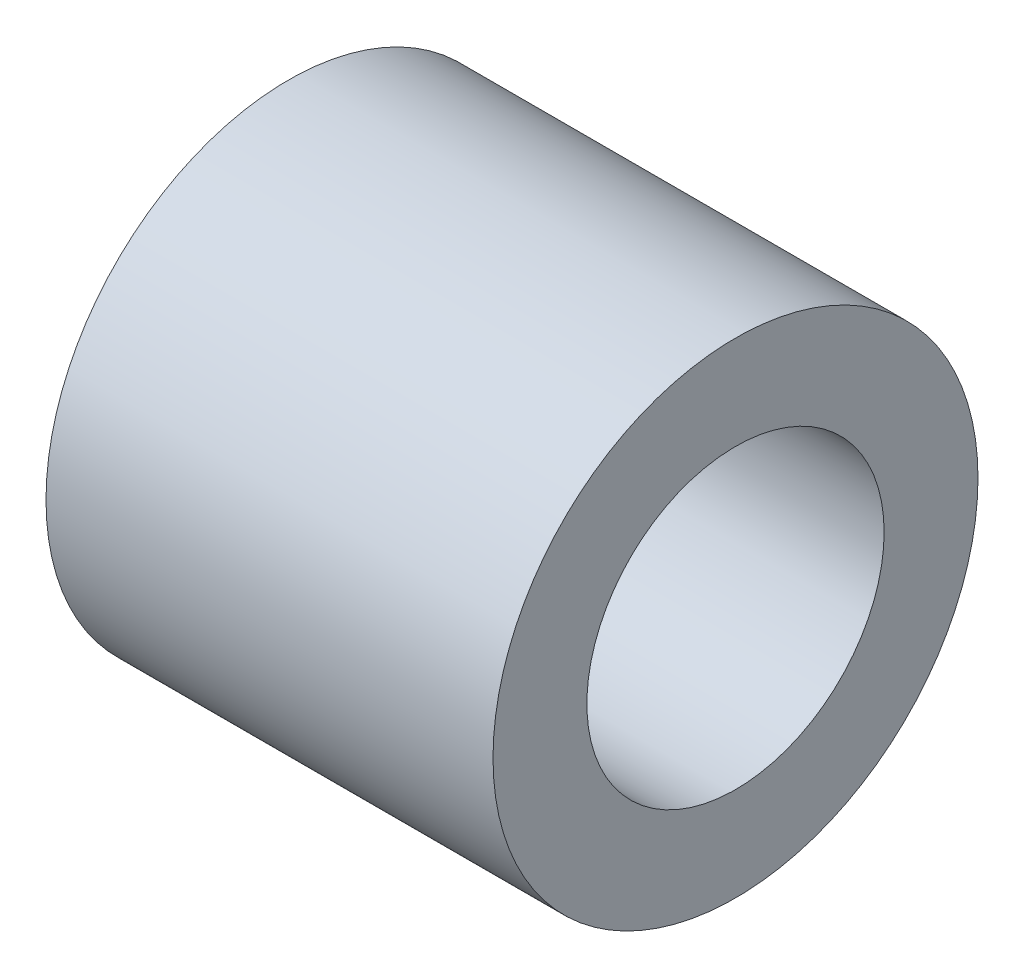
from build123d import *

# Parameters (mm, degrees)
SKETCH1_R           = 10.85
SKETCH1_R_2         = 6.65
BOSS_EXTRUDE1_DEPTH = 20


with BuildPart() as part:
    # Sketch1 → Boss-Extrude1 (new body)
    with BuildSketch(Plane(origin=(0, 0, 0), x_dir=(0, 0, -1), z_dir=(1, 0, 0))):
        Circle(SKETCH1_R)
        Circle(SKETCH1_R_2, mode=Mode.SUBTRACT)
    extrude(amount=BOSS_EXTRUDE1_DEPTH)


solid = part.part
